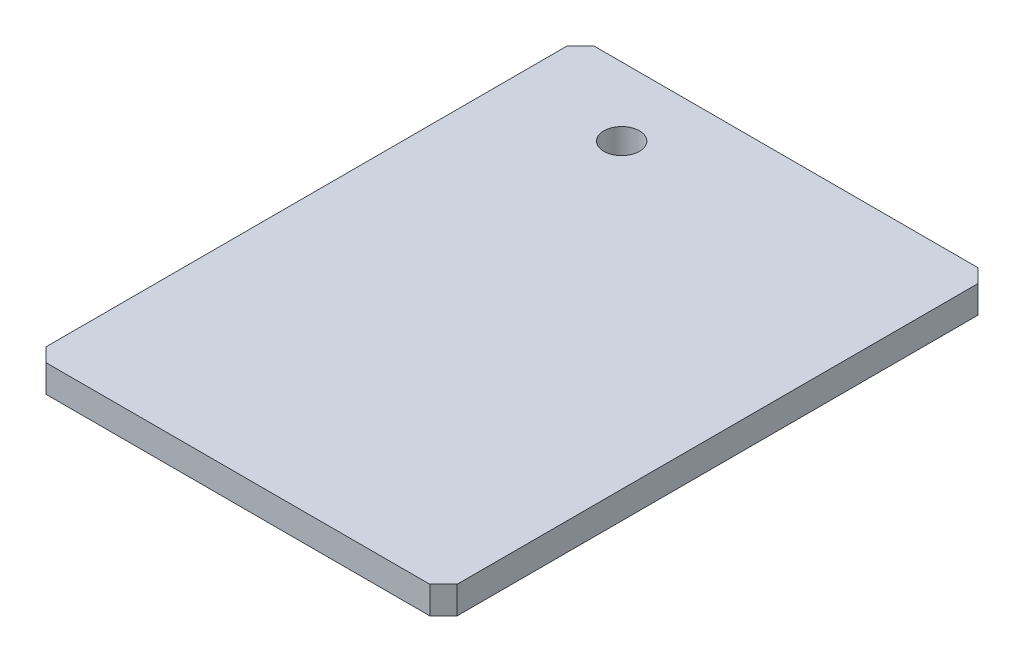
SolidWorks part; units mm, degrees
ref_plane "前视基准面" through (0, 0, 0) normal (0, 0, 1) x (1, 0, 0)
ref_plane "上视基准面" through (0, 0, 0) normal (0, 1, 0) x (1, 0, 0)
ref_plane "右视基准面" through (0, 0, 0) normal (1, 0, 0) x (0, 0, -1)
sketch "草图1" plane through (0, 0, 0) normal (0, 1, 0) x (1, 0, 0)
  line L1 (-150, -200) -> (150, -200)
  line L2 (-150, -200) -> (-150, 200)
  line L3 (-150, 200) -> (150, 200)
  line L4 (150, -200) -> (150, 200)
  line L5 (-150, -200) -> (150, 200) construction
  line L6 (-150, 200) -> (150, -200) construction
  point P0 (0, 0)
  dimension "D1" = 300
  dimension "D2" = 400
extrude "凸台-拉伸1" add sketch "草图1" along normal blind 20
chamfer "倒角1" distance 10 angle 45 4 edges at (150, 10, 200) (-150, 10, 200) (-150, 10, -200) (150, 10, -200)
sketch "草图4" plane through (0, 0, 0) normal (0, -1, 0) x (-1, 0, 0)
  line L0 (-140, 200) -> (140, 200) construction
  line L1 (150, 190) -> (150, -190) construction
  point P0 (70, 150)
  dimension "D1" = 50
  dimension "D2" = 80
hole_wizard "M24 间隙孔1" positions "草图4" profile "草图3" hole size "M24" standard "GB" end condition through all
sketch "草图3" plane through (-70, 0, -150) normal (1, 0, 0) x (0, 0, -1)
  line L0 (0, 0) -> (0, 20)
  line L1 (0, 20) -> (13, 20)
  line L2 (13, 20) -> (13, 0)
  line L5 (13, 0) -> (0, 0)
  line L11 (0, -6.35) -> (0, 107.95) construction
  dimension "通孔孔直径" = 26
  dimension "通孔孔深度" = 20
